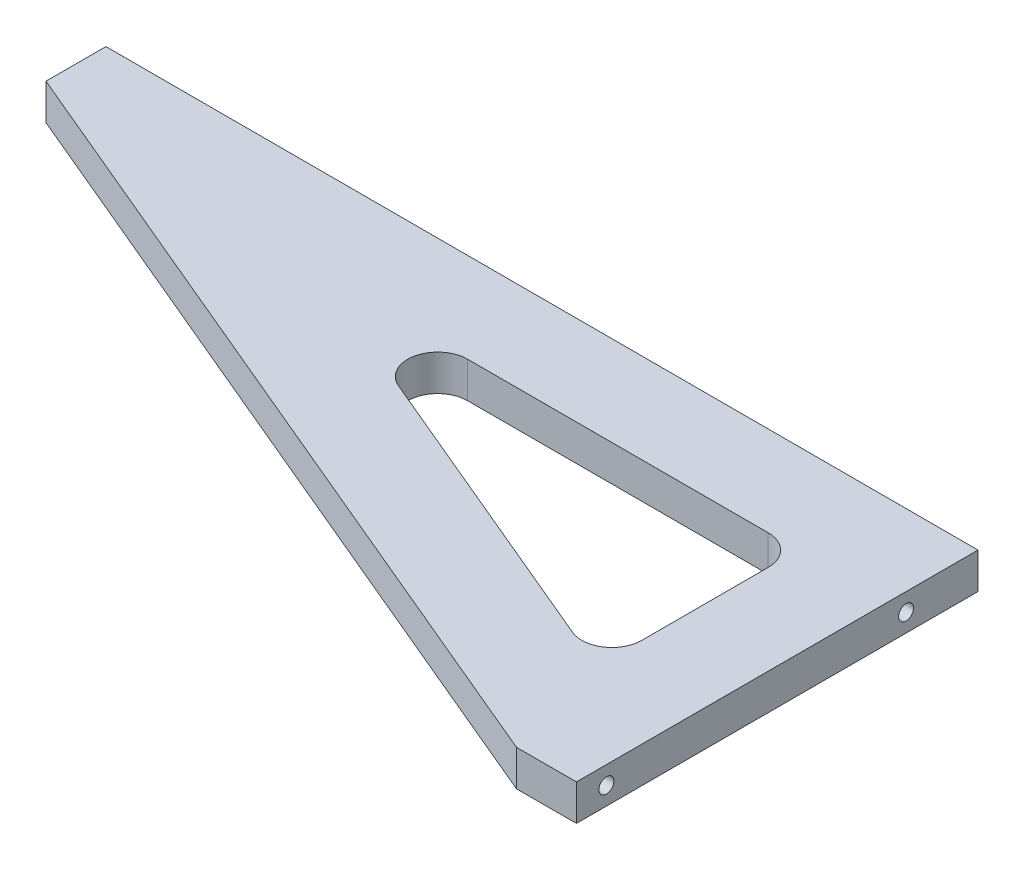
from build123d import *

# Parameters (mm, degrees)
SKETCH_1_W             = 291
SKETCH_1_H             = 134
EXTRUDE_1_DEPTH        = 6
CUT_EXTRUDE_1_DEPTH    = 161.633900532
HOLE_WIZARD_M6_1_D     = 5
HOLE_WIZARD_M6_1_DEPTH = 15
HOLE_WIZARD_M6_1_TIP   = 1.502151548
HOLE_WIZARD_M6_2_D     = 5
HOLE_WIZARD_M6_2_DEPTH = 15
HOLE_WIZARD_M6_2_TIP   = 1.502151548


with BuildPart() as part:
    # 草图1 → 凸台-拉伸1 (new, symmetric)
    with BuildSketch(Plane(origin=(0, 0, 0), x_dir=(1, 0, 0), z_dir=(0, 1, 0))):
        Rectangle(SKETCH_1_W, SKETCH_1_H)
    extrude(amount=EXTRUDE_1_DEPTH, both=True)

    # 草图2 → 切除-拉伸1 (cut, through all)
    with BuildSketch(Plane(origin=(0, 6, 0), x_dir=(1, 0, 0), z_dir=(0, 1, 0))):
        Polygon((-145.5, -67), (125.5, -67), (-145.5, 47), align=None)
        with BuildLine():
            Line((115.5, -15.191630897), (115.5, 27))
            ThreePointArc((115.5, 27), (112.571067812, 34.071067812), (105.5, 37))
            Line((105.5, 37), (5.202351114, 37))
            ThreePointArc((5.202351114, 37), (-4.600106168, 28.977834985), (1.324822524, 17.782366246))
            Line((1.324822524, 17.782366246), (101.62247141, -24.409264651))
            ThreePointArc((101.62247141, -24.409264651), (111.032843487, -23.521555443), (115.5, -15.191630897))
        make_face()
    extrude(amount=-CUT_EXTRUDE_1_DEPTH, mode=Mode.SUBTRACT)

    # M6 螺纹孔1
    with Locations(Plane(origin=(145.5, 0, 0), x_dir=(0, 0, -1), z_dir=(1, 0, 0))):
        with Locations((-57, 0), (43, 0)):
            Hole(HOLE_WIZARD_M6_1_D / 2, depth=HOLE_WIZARD_M6_1_DEPTH)
            with Locations((0, 0, -(HOLE_WIZARD_M6_1_DEPTH + HOLE_WIZARD_M6_1_TIP / 2))):  # 118° drill point
                Cone(0, HOLE_WIZARD_M6_1_D / 2, HOLE_WIZARD_M6_1_TIP, mode=Mode.SUBTRACT)

    # M6 螺纹孔2
    with Locations(Plane(origin=(0, 0, -67), x_dir=(-1, 0, 0), z_dir=(0, 0, -1))):
        with Locations((135.5, 0), (25.5, 0), (-84.5, 0)):
            Hole(HOLE_WIZARD_M6_2_D / 2, depth=HOLE_WIZARD_M6_2_DEPTH)
            with Locations((0, 0, -(HOLE_WIZARD_M6_2_DEPTH + HOLE_WIZARD_M6_2_TIP / 2))):  # 118° drill point
                Cone(0, HOLE_WIZARD_M6_2_D / 2, HOLE_WIZARD_M6_2_TIP, mode=Mode.SUBTRACT)


solid = part.part
